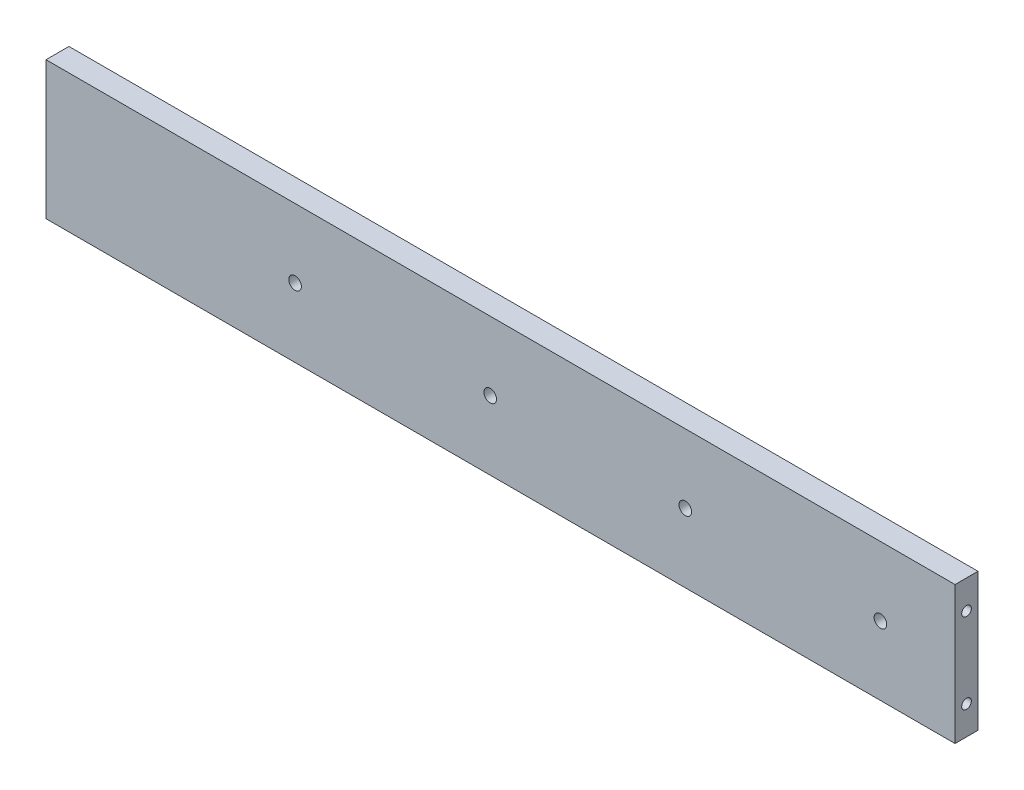
from build123d import *

# Parameters (mm, degrees)
SKETCH1_W                                            = 396
SKETCH1_H                                            = 60
BOSS_EXTRUDE1_DEPTH                                  = 10
HOLE_SIZE_PER_SOCKET_HEAD_CAP_SCREW_TYPE_D           = 5.5
HOLE_SIZE_PER_SOCKET_HEAD_CAP_SCREW_TYPE_CBORE_D     = 10
HOLE_SIZE_PER_SOCKET_HEAD_CAP_SCREW_TYPE_CBORE_DEPTH = 5.7
M5_TAPPED_HOLE1_AT_2_COUNT                           = 2
M5_TAPPED_HOLE1_AT_2_PITCH                           = 35


with BuildPart() as part:
    # Sketch1 → Boss-Extrude1 (new body)
    with BuildSketch(Plane.XY):
        Rectangle(SKETCH1_W, SKETCH1_H)
    extrude(amount=BOSS_EXTRUDE1_DEPTH)

    # Hole size per socket head cap screw type 1 (through all)
    with Locations(Plane(origin=(0, 0, 0), x_dir=(-1, 0, 0), z_dir=(0, 0, -1))):
        with Locations((89.5, 0), (4.5, 0), (-80.5, 0), (-165.5, 0)):
            CounterBoreHole(HOLE_SIZE_PER_SOCKET_HEAD_CAP_SCREW_TYPE_D / 2, HOLE_SIZE_PER_SOCKET_HEAD_CAP_SCREW_TYPE_CBORE_D / 2, HOLE_SIZE_PER_SOCKET_HEAD_CAP_SCREW_TYPE_CBORE_DEPTH)

    # Sketch4 → M5 Tapped Hole1 (revolve, cut)
    with BuildSketch(Plane(origin=(-198, 17.5, 5), x_dir=(0, 0, 1), z_dir=(0, 1, 0))):
        Polygon((0, 0), (0, 13.6618073), (2.1, 12.4), (2.1, 0), align=None)
    m5_tapped_hole1 = revolve(axis=Axis((-204.35, 17.5, 5), (1, 0, 0)), mode=Mode.SUBTRACT)

    # M5 Tapped Hole1 at 2: M5 Tapped Hole1 ×2
    with Locations(*[(0, -i * M5_TAPPED_HOLE1_AT_2_PITCH, 0) for i in range(1, M5_TAPPED_HOLE1_AT_2_COUNT)]):
        add(m5_tapped_hole1, mode=Mode.SUBTRACT)

    # Mirror1: M5 Tapped Hole1 across plane
    add(m5_tapped_hole1.mirror(Plane(origin=(0, 0, 0), x_dir=(0, 0, 1), z_dir=(1, 0, 0))), mode=Mode.SUBTRACT)

    # Mirror1 copy 1 sketch → Mirror1 copy 1 (revolve, cut)
    with BuildSketch(Plane(origin=(198, -17.5, 5), x_dir=(0, 0, 1), z_dir=(0, 1, 0))):
        Polygon((0, 0), (0, -13.6618073), (2.1, -12.4), (2.1, 0), align=None)
    revolve(axis=Axis((204.35, -17.5, 5), (1, 0, 0)), mode=Mode.SUBTRACT)


solid = part.part
